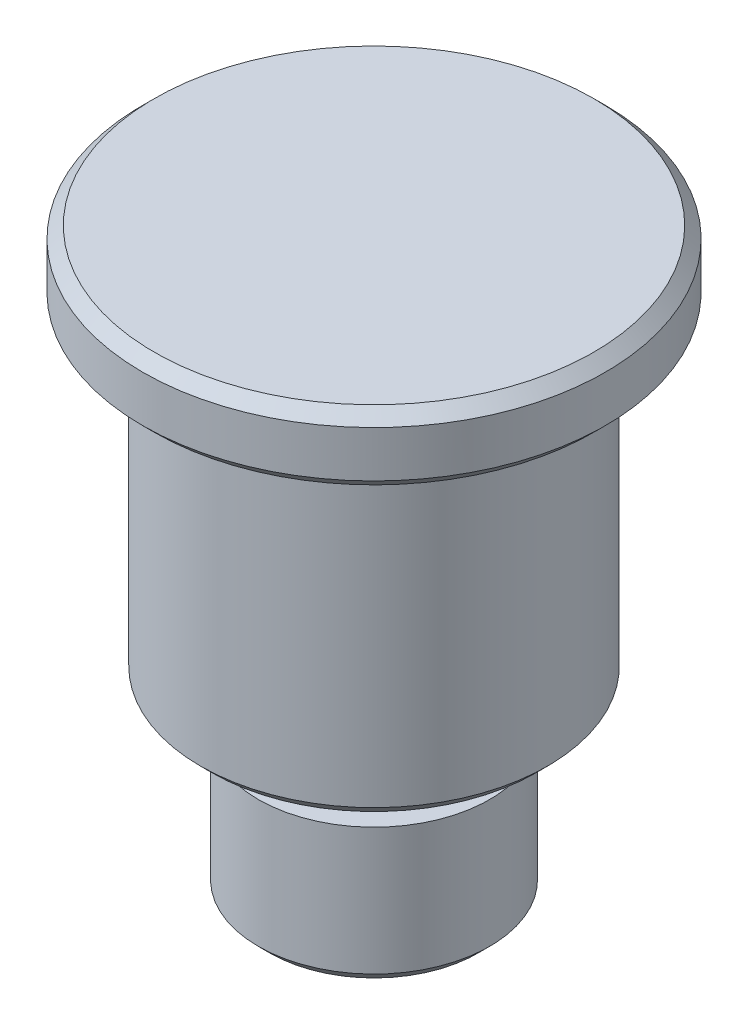
from build123d import *

# Parameters (mm, degrees)
CHAMFER1_SIZE = 0.5


with BuildPart() as part:
    # Sketch1 → Revolve1 (revolve)
    with BuildSketch(Plane(origin=(0, 0, 0), x_dir=(0, 0, -1), z_dir=(1, 0, 0)), mode=Mode.PRIVATE) as revolve1_sk:
        Polygon((0, 0), (10, 0), (10, -3), (7.5, -3), (7.5, -17), (4, -17), (4, -19), (5, -19), (5, -25), (0, -25), align=None)
    revolve(revolve1_sk.sketch.rotate(Axis((0, 0, 0), (0, -1, 0)), 180), axis=Axis((0, 0, 0), (0, -1, 0)))

    # Chamfer1
    chamfer1_edges = [part.edges().sort_by_distance(p)[0] for p in [
        (0, -17, -7.5),
        (0, -3, -10),
        (0, 0, -10),
        (0, -25, -5),
    ]]
    chamfer(chamfer1_edges, length=CHAMFER1_SIZE)


solid = part.part
